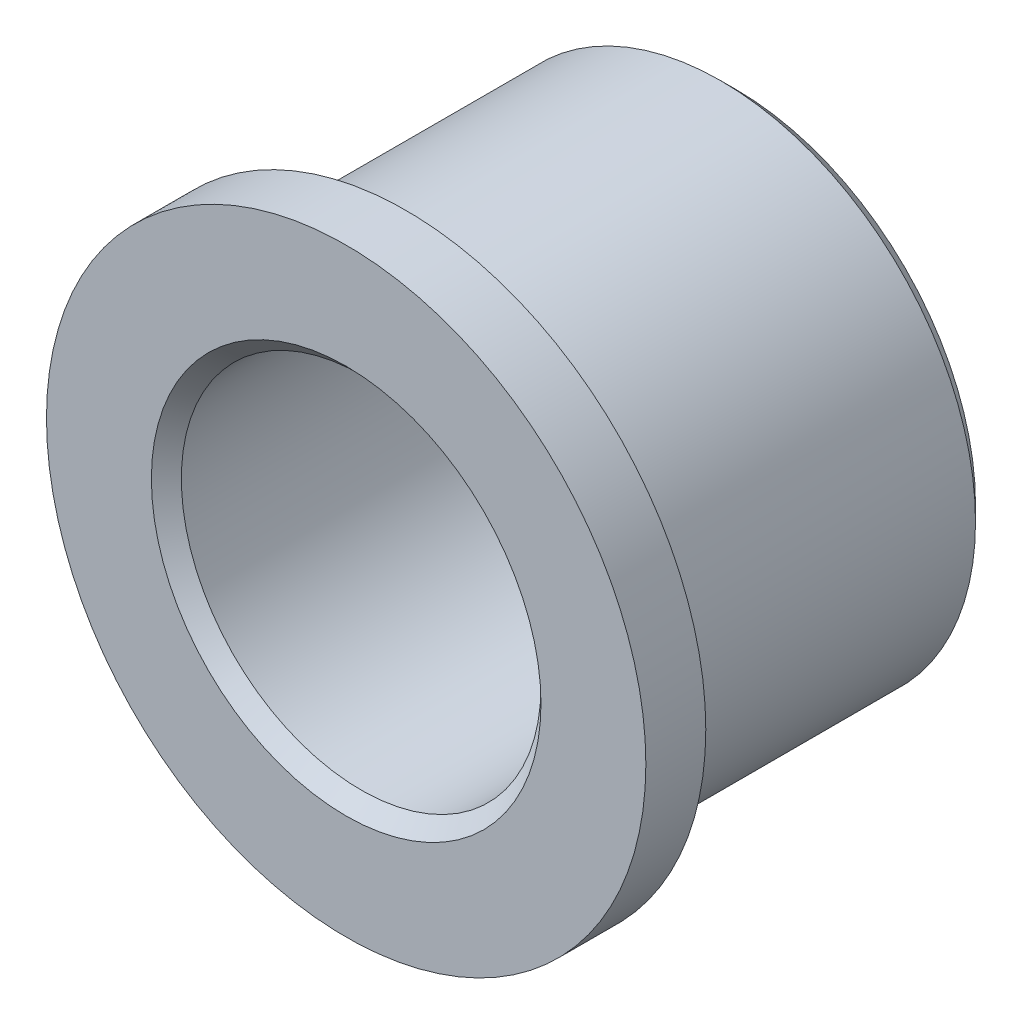
SolidWorks part; units mm, degrees
ref_plane "Front Plane" through (0, 0, 0) normal (0, 0, 1) x (1, 0, 0)
ref_plane "Top Plane" through (0, 0, 0) normal (0, 1, 0) x (1, 0, 0)
ref_plane "Right Plane" through (0, 0, 0) normal (1, 0, 0) x (0, 0, -1)
other "Configuration Table"
sketch "Sketch1" plane through (0, 0, 0) normal (0, 0, 1) x (1, 0, 0)
  circle A0 centre (0, 0) radius 8.5
  dimension "D1" = 17
extrude "Boss-Extrude1" add sketch "Sketch1" along normal blind 13
sketch "Sketch2" plane through (0, 0, 13) normal (0, 0, 1) x (1, 0, 0)
  circle A0 centre (0, 0) radius 10
  dimension "D1" = 20
extrude "Boss-Extrude2" add sketch "Sketch2" against normal blind 2
sketch "Sketch3" plane through (0, 0, 0) normal (0, 0, -1) x (-1, 0, 0)
  circle A0 centre (0, 0) radius 6
  dimension "D1" = 12
extrude "Cut-Extrude1" cut sketch "Sketch3" against normal blind 25
chamfer "Chamfer1" distance 0.5 angle 45 3 edges at (6, 0, 13) (-6, 0, 0) (8.5, 0, 0)
